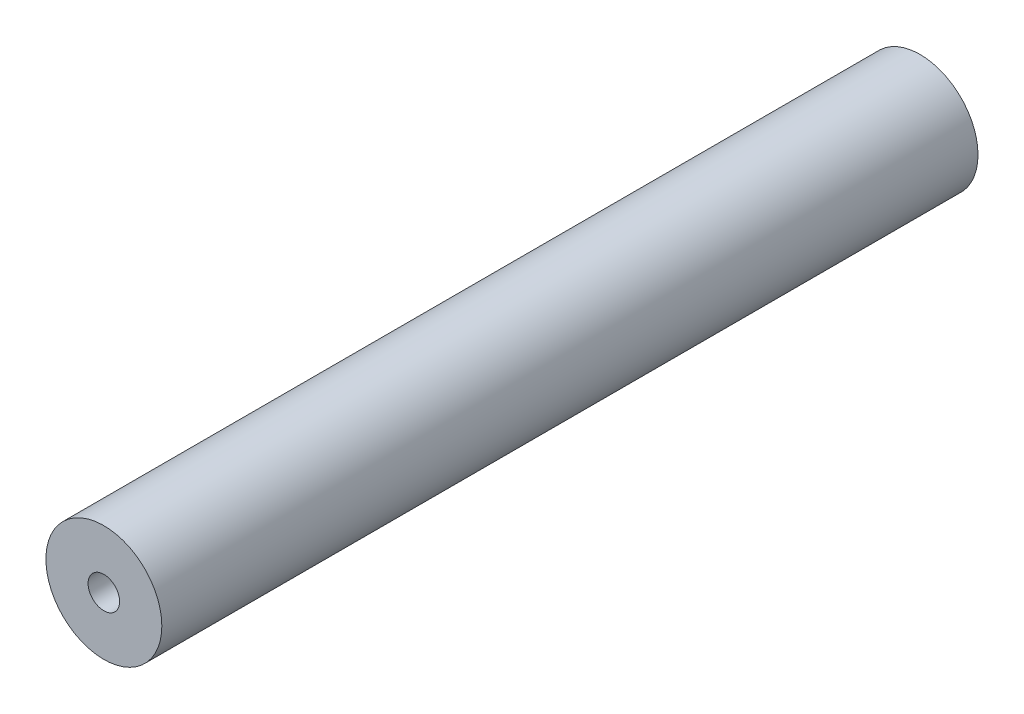
from build123d import *

# Parameters (mm, degrees)
SKETCH_1_R             = 12.5
EXTRUDE_1_DEPTH        = 176
HOLE_WIZARD_M8_1_D     = 6.8
HOLE_WIZARD_M8_1_DEPTH = 19.75
HOLE_WIZARD_M8_1_TIP   = 2.042926105
HOLE_WIZARD_M8_2_D     = 6.8
HOLE_WIZARD_M8_2_DEPTH = 19.75
HOLE_WIZARD_M8_2_TIP   = 2.042926105


with BuildPart() as part:
    # 草图1 → 凸台-拉伸1 (new body)
    with BuildSketch(Plane.XY):
        Circle(SKETCH_1_R)
    extrude(amount=EXTRUDE_1_DEPTH)

    # M8 螺纹孔1
    with Locations(Plane(origin=(0, 0, 0), x_dir=(-1, 0, 0), z_dir=(0, 0, -1))):
        with Locations((0, 0)):
            Hole(HOLE_WIZARD_M8_1_D / 2, depth=HOLE_WIZARD_M8_1_DEPTH)
            with Locations((0, 0, -(HOLE_WIZARD_M8_1_DEPTH + HOLE_WIZARD_M8_1_TIP / 2))):  # 118° drill point
                Cone(0, HOLE_WIZARD_M8_1_D / 2, HOLE_WIZARD_M8_1_TIP, mode=Mode.SUBTRACT)

    # M8 螺纹孔2
    with Locations(Plane.XY.offset(176)):
        with Locations((0, 0)):
            Hole(HOLE_WIZARD_M8_2_D / 2, depth=HOLE_WIZARD_M8_2_DEPTH)
            with Locations((0, 0, -(HOLE_WIZARD_M8_2_DEPTH + HOLE_WIZARD_M8_2_TIP / 2))):  # 118° drill point
                Cone(0, HOLE_WIZARD_M8_2_D / 2, HOLE_WIZARD_M8_2_TIP, mode=Mode.SUBTRACT)


solid = part.part
